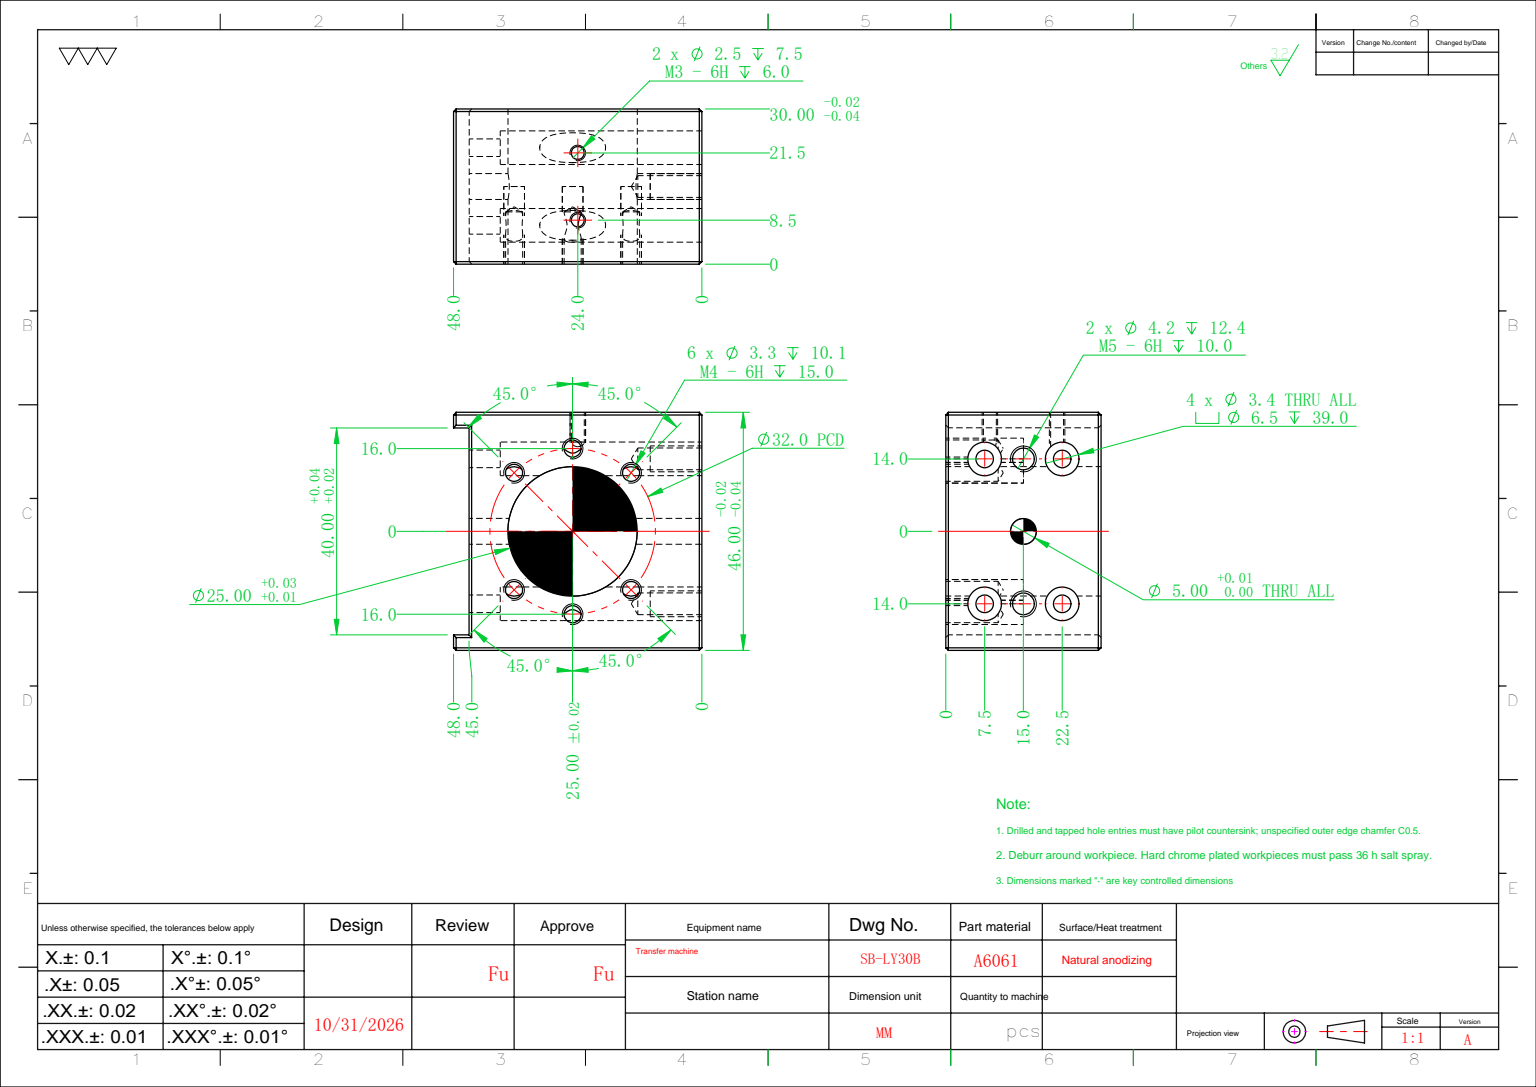
from build123d import *

# Parameters (mm, degrees)
SKETCH_1_W                   = 46
SKETCH_1_H                   = 48
EXTRUDE_1_DEPTH              = 30
SKETCH_2_W                   = 40
SKETCH_2_H                   = 3
CUT_EXTRUDE_1_DEPTH          = 45.777226354
HOLE_WIZARD_M3_1_D           = 3.4
HOLE_WIZARD_M3_1_CBORE_D     = 6.5
HOLE_WIZARD_M3_1_CBORE_DEPTH = 39
SKETCH_5_R                   = 12.5
CUT_EXTRUDE_2_DEPTH          = 45.777226354
MM_1_D                       = 5
CHAMFER_1_SIZE               = 0.5
HOLE_WIZARD_M5_1_D           = 4.2
HOLE_WIZARD_M5_1_DEPTH       = 12.4
HOLE_WIZARD_M5_1_TIP         = 1.2618073
HOLE_WIZARD_M3_2_D           = 2.5
HOLE_WIZARD_M3_2_DEPTH       = 7.5
HOLE_WIZARD_M3_2_TIP         = 0.751075774
HOLE_WIZARD_M4_1_D           = 3.3
HOLE_WIZARD_M4_1_DEPTH       = 10.1
HOLE_WIZARD_M4_1_TIP         = 0.991420021


with BuildPart() as part:
    # 草图1 → 凸台-拉伸1 (new body)
    with BuildSketch(Plane.XY):
        Rectangle(SKETCH_1_W, SKETCH_1_H)
    extrude(amount=EXTRUDE_1_DEPTH)

    # 草图2 → 切除-拉伸1 (cut, through all)
    with BuildSketch(Plane.XY.offset(30)):
        with Locations((0, -22.5)):
            Rectangle(SKETCH_2_W, SKETCH_2_H)
    extrude(amount=-CUT_EXTRUDE_1_DEPTH, mode=Mode.SUBTRACT)

    # M3 六角凹头螺钉的柱形沉头孔1 (through all)
    with Locations(Plane(origin=(0, 24, 0), x_dir=(1, 0, 0), z_dir=(0, 1, 0))):
        with Locations((-14, -7.5), (14, -7.5), (14, -22.5), (-14, -22.5)):
            CounterBoreHole(HOLE_WIZARD_M3_1_D / 2, HOLE_WIZARD_M3_1_CBORE_D / 2, HOLE_WIZARD_M3_1_CBORE_DEPTH)

    # 草图5 → 切除-拉伸2 (cut, through all)
    with BuildSketch(Plane.XY.offset(30)):
        with Locations((0, -1)):
            Circle(SKETCH_5_R)
    extrude(amount=-CUT_EXTRUDE_2_DEPTH, mode=Mode.SUBTRACT)

    # 大小mm 暗销孔1 (through all)
    with Locations(Plane(origin=(0, 24, 0), x_dir=(1, 0, 0), z_dir=(0, 1, 0))):
        with Locations((0, -15)):
            Hole(MM_1_D / 2)

    # 倒角1
    chamfer_1_edges = [part.edges().sort_by_distance(p)[0] for p in [
        (-23, 0, 30),
        (-21.5, -24, 30),
        (21.5, -24, 0),
        (21.5, -24, 30),
        (-20, -22.5, 0),
        (0, -21, 0),
        (20, -22.5, 0),
        (-20, -22.5, 30),
        (20, -22.5, 30),
        (0, -21, 30),
        (23, 0, 30),
        (-21.5, -24, 0),
        (-23, 0, 0),
        (0, 24, 0),
        (23, 0, 0),
        (0, 24, 30),
        (23, -24, 15),
        (-23, -24, 15),
        (-23, 24, 15),
        (23, 24, 15),
    ]]
    chamfer(chamfer_1_edges, length=CHAMFER_1_SIZE)

    # M5 螺纹孔1
    with Locations(Plane(origin=(0, 24, 0), x_dir=(1, 0, 0), z_dir=(0, 1, 0))):
        with Locations((-14, -15), (14, -15)):
            Hole(HOLE_WIZARD_M5_1_D / 2, depth=HOLE_WIZARD_M5_1_DEPTH)
            with Locations((0, 0, -(HOLE_WIZARD_M5_1_DEPTH + HOLE_WIZARD_M5_1_TIP / 2))):  # 118° drill point
                Cone(0, HOLE_WIZARD_M5_1_D / 2, HOLE_WIZARD_M5_1_TIP, mode=Mode.SUBTRACT)

    # M3 螺纹孔2
    with Locations(Plane(origin=(23, 0, 0), x_dir=(0, 0, -1), z_dir=(1, 0, 0))):
        with Locations((-21.5, 0), (-8.5, 0)):
            Hole(HOLE_WIZARD_M3_2_D / 2, depth=HOLE_WIZARD_M3_2_DEPTH)
            with Locations((0, 0, -(HOLE_WIZARD_M3_2_DEPTH + HOLE_WIZARD_M3_2_TIP / 2))):  # 118° drill point
                Cone(0, HOLE_WIZARD_M3_2_D / 2, HOLE_WIZARD_M3_2_TIP, mode=Mode.SUBTRACT)

    # M4 螺纹孔1
    with Locations(Plane(origin=(0, 0, 0), x_dir=(-1, 0, 0), z_dir=(0, 0, -1))):
        with Locations((-16, -1), (-11.313708499, 10.313708499), (11.313708499, 10.313708499), (16, -1), (11.313708499, -12.313708499), (-11.313708499, -12.313708499)):
            Hole(HOLE_WIZARD_M4_1_D / 2, depth=HOLE_WIZARD_M4_1_DEPTH)
            with Locations((0, 0, -(HOLE_WIZARD_M4_1_DEPTH + HOLE_WIZARD_M4_1_TIP / 2))):  # 118° drill point
                Cone(0, HOLE_WIZARD_M4_1_D / 2, HOLE_WIZARD_M4_1_TIP, mode=Mode.SUBTRACT)


solid = part.part
